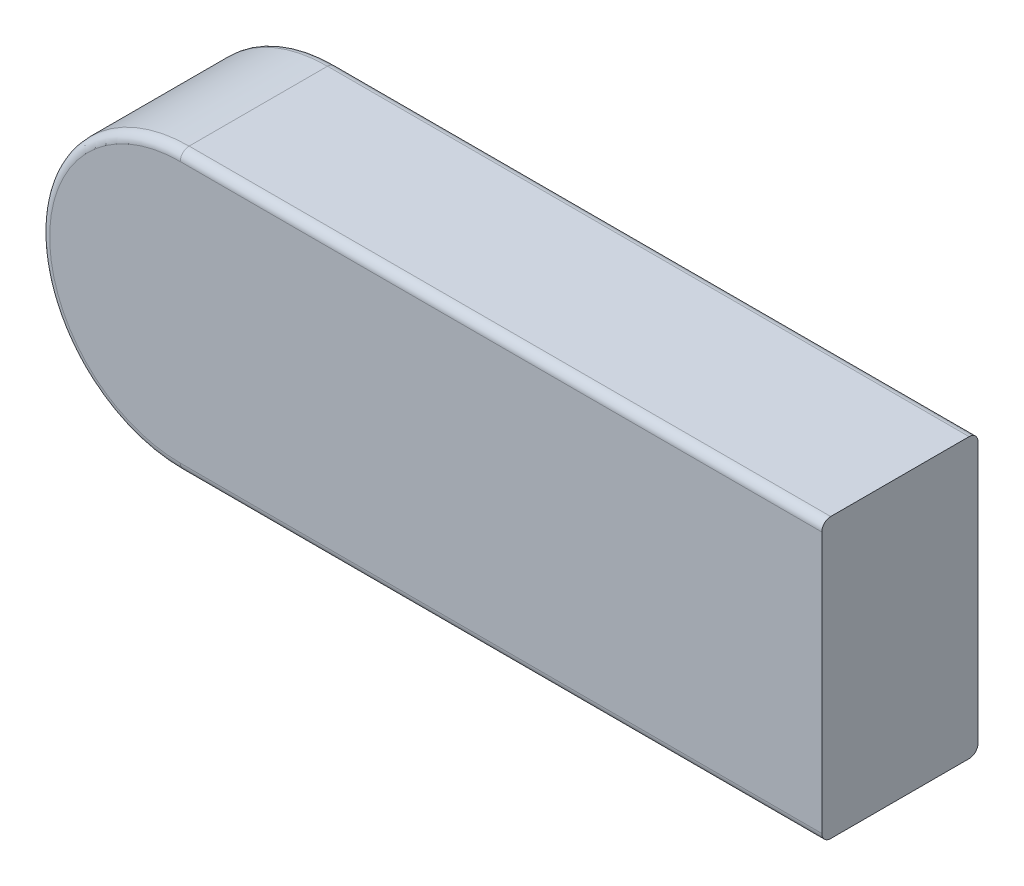
SolidWorks part; units mm, degrees
ref_plane "基准面1" through (0, 0, 0) normal (0, 0, 1) x (1, 0, 0)
ref_plane "基准面2" through (0, 0, 0) normal (0, 1, 0) x (1, 0, 0)
ref_plane "基准面3" through (0, 0, 0) normal (1, 0, 0) x (0, 0, -1)
sketch "尺寸草图" plane through (0, 0, 0) normal (0, 0, 1) x (1, 0, 0)
  line L0 (-35, 0) -> (35, 0) construction
  point P3 (-14, 0)
  point P4 (-0.8, 0)
  point P5 (0, 0)
  point P8 (-25, 0)
  point P11 (0, 0)
sketch "草图1" plane through (0, 0, 0) normal (0, 0, 1) x (1, 0, 0)
  line L0 (-28.0599, 0) -> (30.562, 0) construction
  line L1 (-9, 12.5) -> (48.5, 12.5)
  line L2 (-9, -12.5) -> (48.5, -12.5)
  line L3 (0, 2.9108) -> (0, -2.1805) construction
  line L4 (48.5, 12.5) -> (48.5, -12.5)
  arc A0 (-9, 12.5) -> (-9, -12.5) centre (-9, 0) ccw
extrude "基体-拉伸" add sketch "草图1" along normal blind 14
fillet "圆角1" radius 0.8 6 edges at (-21.5, 0, 14) (19.75, -12.5, 14) (19.75, -12.5, 0) (-21.5, 0, 0) (19.75, 12.5, 0) (19.75, 12.5, 14)
equation "\"D3@草图1\" = \"L@尺寸草图\""
equation "\"D1@草图1\" = \"b@尺寸草图\" / 2"
equation "\"D1@圆角1\" = \"r@尺寸草图\""
equation "\"D1@基体-拉伸\" = \"h@尺寸草图\""
